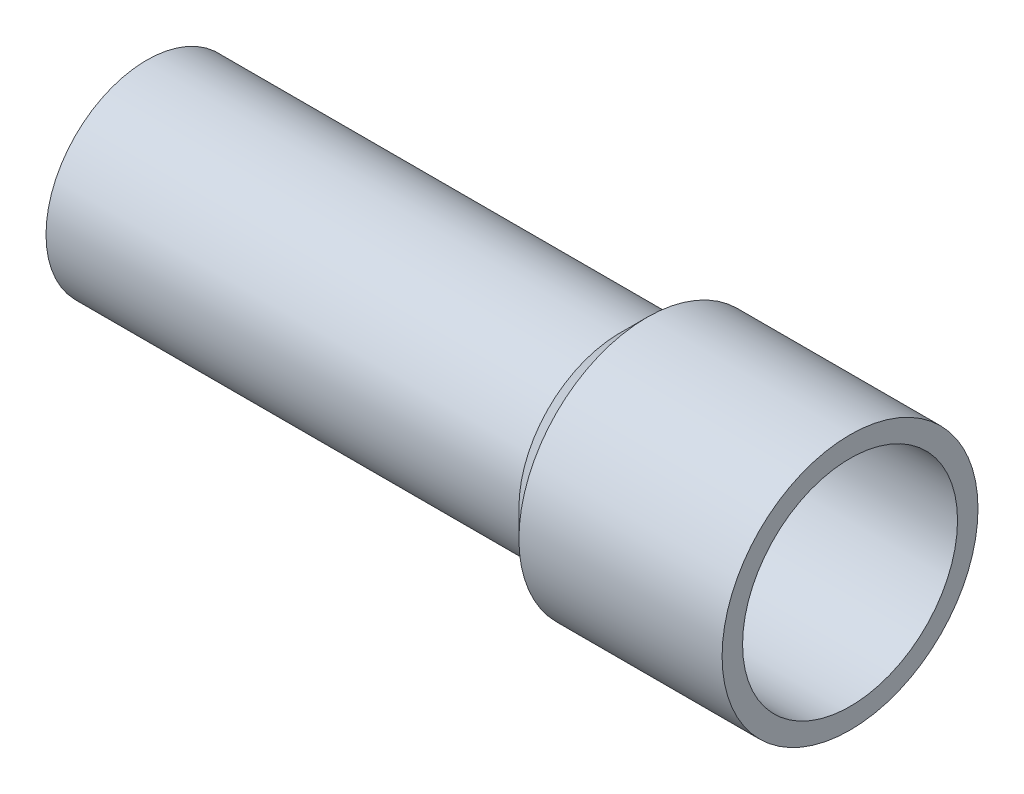
SolidWorks part; units mm, degrees
material "铜"
ref_plane "Front Plane" through (0, 0, 0) normal (0, 0, 1) x (1, 0, 0)
ref_plane "Top Plane" through (0, 0, 0) normal (0, 1, 0) x (1, 0, 0)
ref_plane "Right Plane" through (0, 0, 0) normal (1, 0, 0) x (0, 0, -1)
sketch "Sketch1" plane through (0, 0, 0) normal (0, 0, 1) x (1, 0, 0)
  line L0 (0, 1.97) -> (9.24, 1.97)
  line L1 (9.24, 1.97) -> (9.77, 2.5)
  line L2 (9.77, 2.5) -> (13.74, 2.5)
  line L3 (0, 0) -> (18.4989, 0) construction
  line L4 (0, 1.57) -> (9.4057, 1.57)
  line L5 (9.4057, 1.57) -> (9.9357, 2.1)
  line L6 (9.9357, 2.1) -> (13.74, 2.1)
  line L7 (0, 1.57) -> (0, 1.97)
  line L8 (13.74, 2.1) -> (13.74, 2.5)
  dimension "D1" = 4.5
  dimension "D2" = 5
  dimension "D3" = 13.74
  dimension "D4" = 3.94
  dimension "D5" = 135
  dimension "D6" = 0.4
revolve "Revolve1" add sketch "Sketch1" angle 360 about L3
